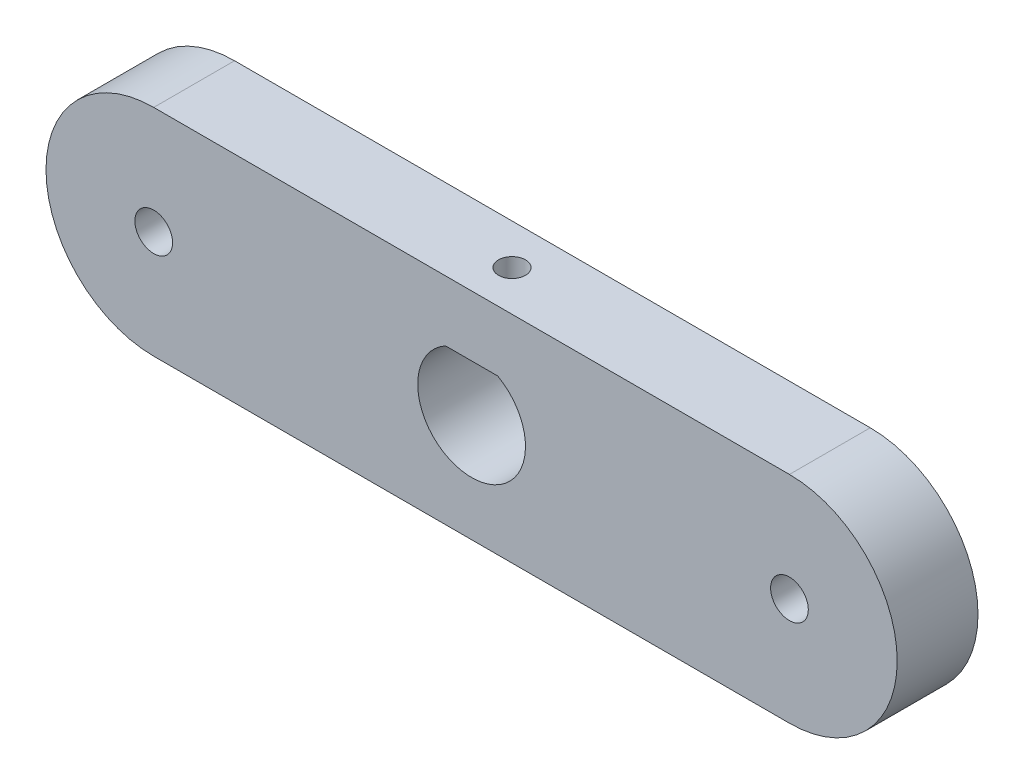
from build123d import *

# Parameters (mm, degrees)
SKETCH_1_R          = 4
EXTRUDE_1_DEPTH     = 6
SKETCH_2_R          = 1.4
CUT_EXTRUDE_1_DEPTH = 34.144531977
SKETCH_3_R          = 1
CUT_EXTRUDE_2_DEPTH = 5
SKETCH_4_W          = 4.960231778
SKETCH_4_H          = 1
EXTRUDE_2_DEPTH     = 6


with BuildPart() as part:
    # 草图1 → 凸台-拉伸1 (new body)
    with BuildSketch(Plane.XY):
        with BuildLine():
            Line((-23.6, 8), (23.6, 8))
            ThreePointArc((23.6, 8), (31.6, 0), (23.6, -8))
            Line((23.6, -8), (-23.6, -8))
            ThreePointArc((-23.6, -8), (-31.6, 0), (-23.6, 8))
        make_face()
        Circle(SKETCH_1_R, mode=Mode.SUBTRACT)
    extrude(amount=EXTRUDE_1_DEPTH)

    # 草图2 → 切除-拉伸1 (cut, through all)
    with BuildSketch(Plane.XY.offset(6)):
        with Locations((-23.6, 0)):
            Circle(SKETCH_2_R)
        with Locations((23.6, 0)):
            Circle(SKETCH_2_R)
    extrude(amount=-CUT_EXTRUDE_1_DEPTH, mode=Mode.SUBTRACT)

    # 草图3 → 切除-拉伸2 (cut)
    with BuildSketch(Plane(origin=(0, 8, 0), x_dir=(1, 0, 0), z_dir=(0, 1, 0))):
        with Locations(Location((0, -3, 0), (0, 0, 180))):
            Circle(SKETCH_3_R)
    extrude(amount=-CUT_EXTRUDE_2_DEPTH, mode=Mode.SUBTRACT)

    # 草图4 → 凸台-拉伸2 (add)
    with BuildSketch(Plane(origin=(0, 0, 0), x_dir=(-1, 0, 0), z_dir=(0, 0, -1))):
        with Locations((0, 4)):
            Rectangle(SKETCH_4_W, SKETCH_4_H)
    extrude(amount=-EXTRUDE_2_DEPTH)


solid = part.part
